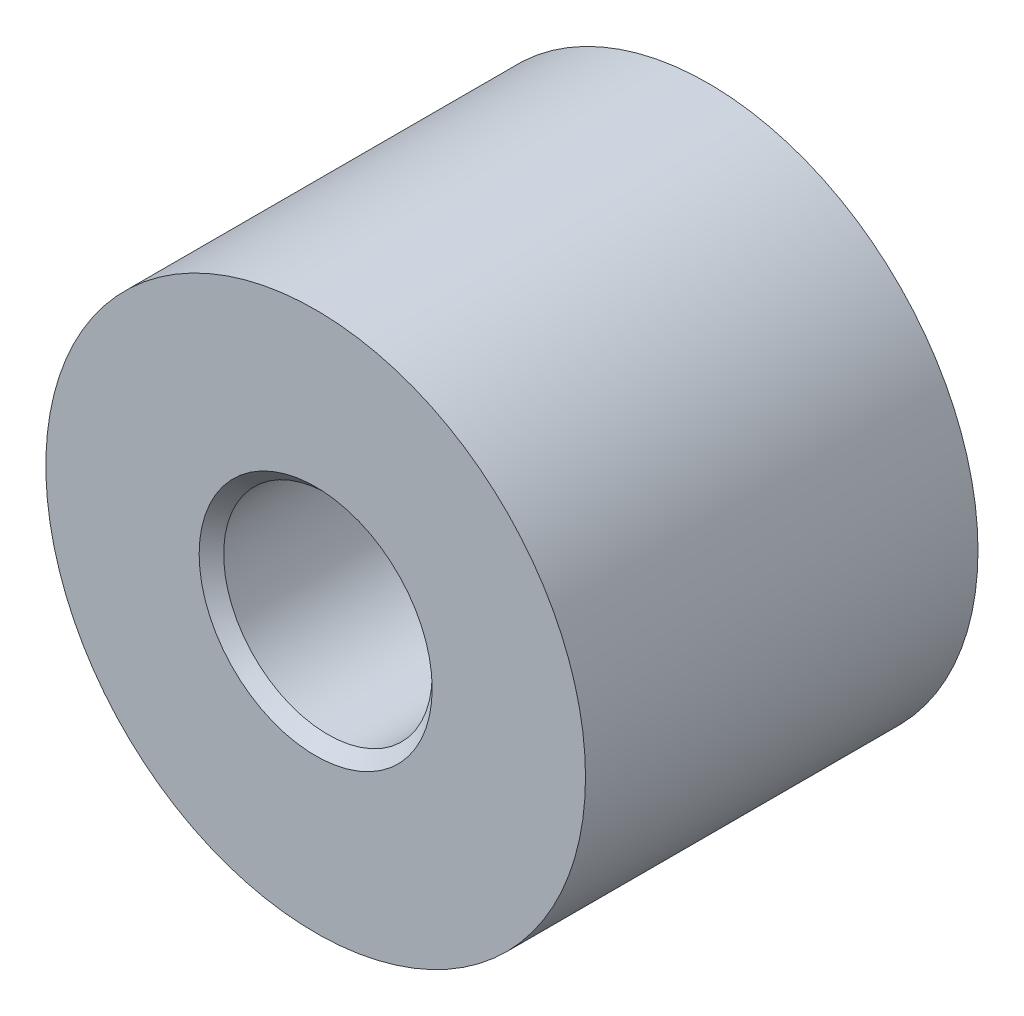
SolidWorks part; units mm, degrees
ref_plane "Front Plane" through (0, 0, 0) normal (0, 0, 1) x (1, 0, 0)
ref_plane "Top Plane" through (0, 0, 0) normal (0, 1, 0) x (1, 0, 0)
ref_plane "Right Plane" through (0, 0, 0) normal (1, 0, 0) x (0, 0, -1)
sketch "Sketch1" plane through (0, 0, 0) normal (0, 0, 1) x (1, 0, 0)
  circle A0 centre (0, 0) radius 11
extrude "Boss-Extrude1" add sketch "Sketch1" along normal blind 16
sketch "Sketch2" plane through (0, 0, 16) normal (0, 0, 1) x (1, 0, 0)
  circle A0 centre (0, 0) radius 4.25
extrude "Cut-Extrude1" cut sketch "Sketch2" against normal blind 16
chamfer "Chamfer1" distance 0.5 angle 45 2 edges at (4.25, 0, 0) (4.25, 0, 16)
